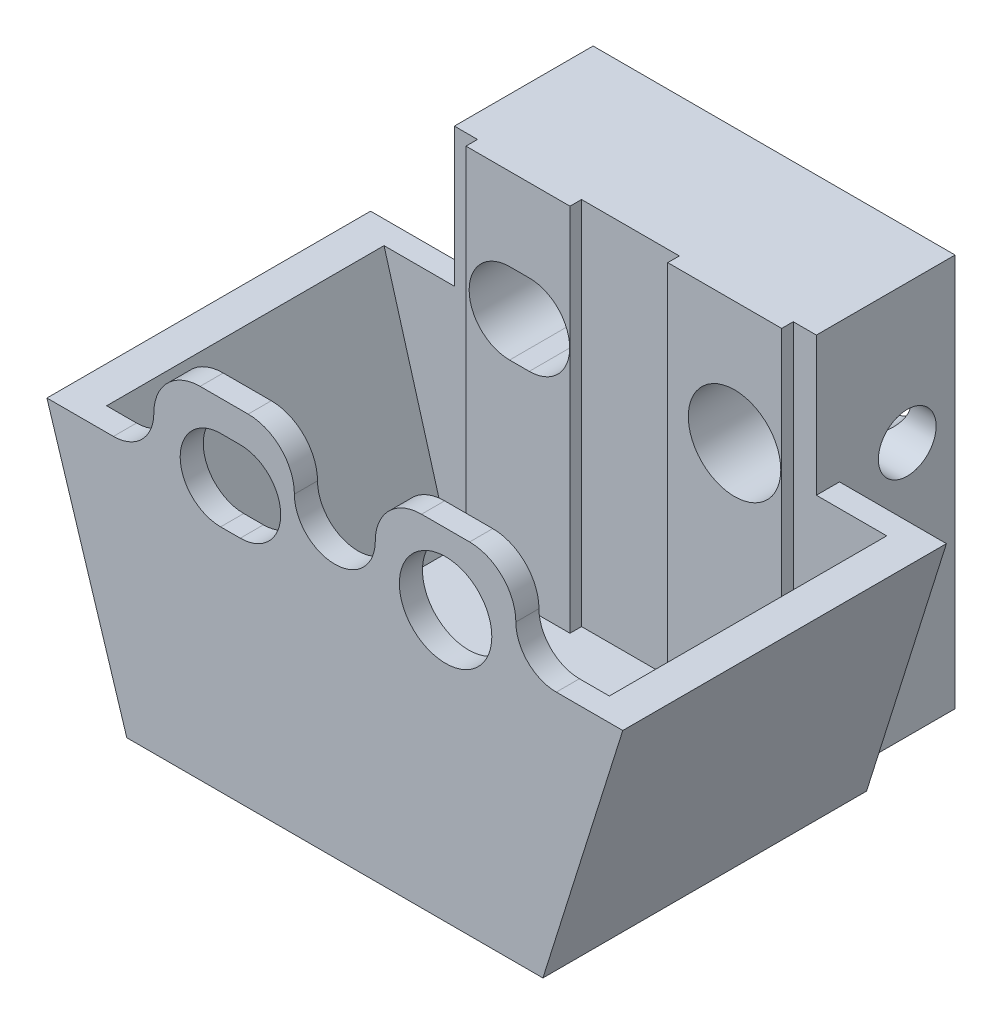
SolidWorks part; units mm, degrees
ref_plane "前视基准面" through (0, 0, 0) normal (0, 0, 1) x (1, 0, 0)
ref_plane "上视基准面" through (0, 0, 0) normal (0, 1, 0) x (1, 0, 0)
ref_plane "右视基准面" through (0, 0, 0) normal (1, 0, 0) x (0, 0, -1)
sketch "草图1" plane through (0, 0, 0) normal (0, 0, 1) x (1, 0, 0)
  line L0 (0, 0) -> (180, 0)
  line L1 (180, 0) -> (180, 220)
  line L2 (0, 0) -> (-69.0989, 220)
  line L3 (-69.0989, 220) -> (-11.5827, 220)
  line L4 (63.4173, 295) -> (105, 295)
  arc A0 (180, 220) -> (145, 255) centre (180, 255) cw
  arc A1 (-11.5827, 220) -> (23.4173, 255) centre (-11.5827, 255) ccw
  arc A2 (23.4173, 255) -> (63.4173, 295) centre (63.4173, 255) cw
  arc A3 (145, 255) -> (105, 295) centre (105, 255) ccw
extrude "凸台-拉伸2" add sketch "草图1" along normal blind 140
sketch3d "3D草图2"
  point P0 (98.2763, 115.3215, 0)
ref_plane "基准面2" through (0, 0, 0) normal (0, 0, -1) x (-1, 0, 0)
sketch "草图5" plane through (0, 0, 0) normal (0, 0, -1) x (-1, 0, 0)
  line L0 (-180, 220) -> (69.0989, 220)
  line L1 (69.0989, 220) -> (0, 0)
  line L2 (0, 0) -> (-180, 0)
  line L3 (-180, 0) -> (-180, 220)
extrude "凸台-拉伸3" add sketch "草图5" along normal blind 140
sketch3d "3D草图3"
  point P0 (84.2298, 295, 74.4461)
ref_plane "基准面3" through (0, 295, 0) normal (0, 1, 0) x (1, 0, 0)
sketch "草图8" plane through (0, 295, 0) normal (0, 1, 0) x (1, 0, 0)
  line L1 (180, -140) -> (180, 0) construction
  line L3 (180, 140) -> (180, 0) construction
  line L4 (180, 120) -> (80, 120)
  line L5 (80, 120) -> (80, -120)
  line L6 (80, -120) -> (180, -120)
  line L7 (180, 120) -> (180, -120)
extrude "切除-拉伸1" cut sketch "草图8" against normal blind 275
sketch3d "3D草图4"
  point P0 (116.3882, 20, -5.7324)
ref_plane "基准面4" through (0, 20, 0) normal (0, 1, 0) x (1, 0, 0)
sketch "草图10" plane through (0, 20, 0) normal (0, 1, 0) x (1, 0, 0)
  line L0 (80, 120) -> (20, 120)
  line L1 (20, 120) -> (20, -120)
  line L2 (20, -120) -> (80, -120)
  line L3 (80, -120) -> (80, 120)
sketch "草图11" plane through (0, 295, 0) normal (0, 1, 0) x (1, 0, 0)
  line L0 (80, 120) -> (80, -120)
  line L1 (80, -120) -> (-59, -120)
  line L2 (-59, -120) -> (-59, 120)
  line L3 (-59, 120) -> (80, 120)
loft "切除-放样4" cut profiles "草图10", "草图11"
mirror "镜向1" about plane through (180, 0, 140) normal (-1, 0, 0) of "切除-放样4", "切除-拉伸1", "凸台-拉伸3", "凸台-拉伸2"
sketch3d "3D草图5"
  point P0 (226.624, 136.3844, -140)
ref_plane "基准面5" through (0, 0, -140) normal (0, 0, -1) x (-1, 0, 0)
sketch "草图12" plane through (0, 0, -140) normal (0, 0, -1) x (-1, 0, 0)
  line L0 (-336.5827, 220) -> (-336.5827, 340)
  line L1 (69.0989, 220) -> (-429.0989, 220) construction
  line L2 (-336.5827, 220) -> (-23.4173, 220)
  line L3 (-336.5827, 340) -> (-23.4173, 340)
  line L4 (-23.4173, 340) -> (-23.4173, 220)
extrude "凸台-拉伸4" add sketch "草图12" along normal blind 100 and the other way blind 20
sketch "草图13" plane through (0, 0, -140) normal (0, 0, -1) x (-1, 0, 0)
  line L0 (-336.5827, 220) -> (-336.5827, 0)
  line L1 (-360, 0) -> (0, 0) construction
  line L2 (-336.5827, 0) -> (-23.4173, 0)
  line L3 (-23.4173, 0) -> (-23.4173, 220)
  line L4 (-23.4173, 220) -> (-336.5827, 220)
extrude "凸台-拉伸5" add sketch "草图13" along normal blind 100
sketch3d "3D草图6"
  point P0 (336.5827, 174.9086, -185.5314)
ref_plane "基准面6" through (336.5827, 0, 0) normal (1, 0, 0) x (0, 0, -1)
sketch "草图14" plane through (336.5827, 0, 0) normal (1, 0, 0) x (0, 0, -1)
  circle A0 centre (198.6209, 220) radius 25
extrude "切除-拉伸2" cut sketch "草图14" against normal through all
sketch3d "3D草图7"
  point P0 (201.9225, 340, -191.4158)
ref_plane "基准面7" through (0, 340, 0) normal (0, 1, 0) x (1, 0, 0)
sketch "草图15" plane through (0, 340, 0) normal (0, 1, 0) x (1, 0, 0)
  line L1 (23.4173, 120) -> (336.5827, 120) construction
  line L2 (43.4173, 120) -> (43.4173, 110)
  line L3 (43.4173, 110) -> (133.4173, 110)
  line L4 (133.4173, 110) -> (133.4173, 120)
  line L5 (280, 120) -> (80, 120) construction
  line L6 (133.4173, 120) -> (43.4173, 120)
  line L7 (316.5827, 120) -> (218, 120)
  line L8 (218, 120) -> (218, 110)
  line L9 (218, 110) -> (316.5827, 110)
  line L10 (316.5827, 110) -> (316.5827, 120)
  point P0 (0, 0)
extrude "凸台-拉伸6" add sketch "草图15" against normal up to surface (320 mm away) contours L2 L3 L4 L6 | L7 L8 L9 L10 up to face at (180, 20, -30)
sketch "草图16" plane through (0, 0, -140) normal (0, 0, -1) x (-1, 0, 0)
  line L2 (-98.1764, 268.6063) -> (-81.1764, 268.6063)
  line L3 (-81.1764, 198.6063) -> (-98.1764, 198.6063)
  circle A0 centre (-275.7914, 233.6063) radius 40
  arc A1 (-81.1764, 268.6063) -> (-81.1764, 198.6063) centre (-81.1764, 233.6063) cw
  arc A2 (-98.1764, 268.6063) -> (-98.1764, 198.6063) centre (-98.1764, 233.6063) ccw
  point P3 (0, 0)
  point P4 (0, 0)
  point P10 (0, 0)
  point P11 (0, 0)
  point P12 (0, 0)
  point P13 (0, 0)
extrude "切除-拉伸3" cut sketch "草图16" against normal through all both and the other way through all
